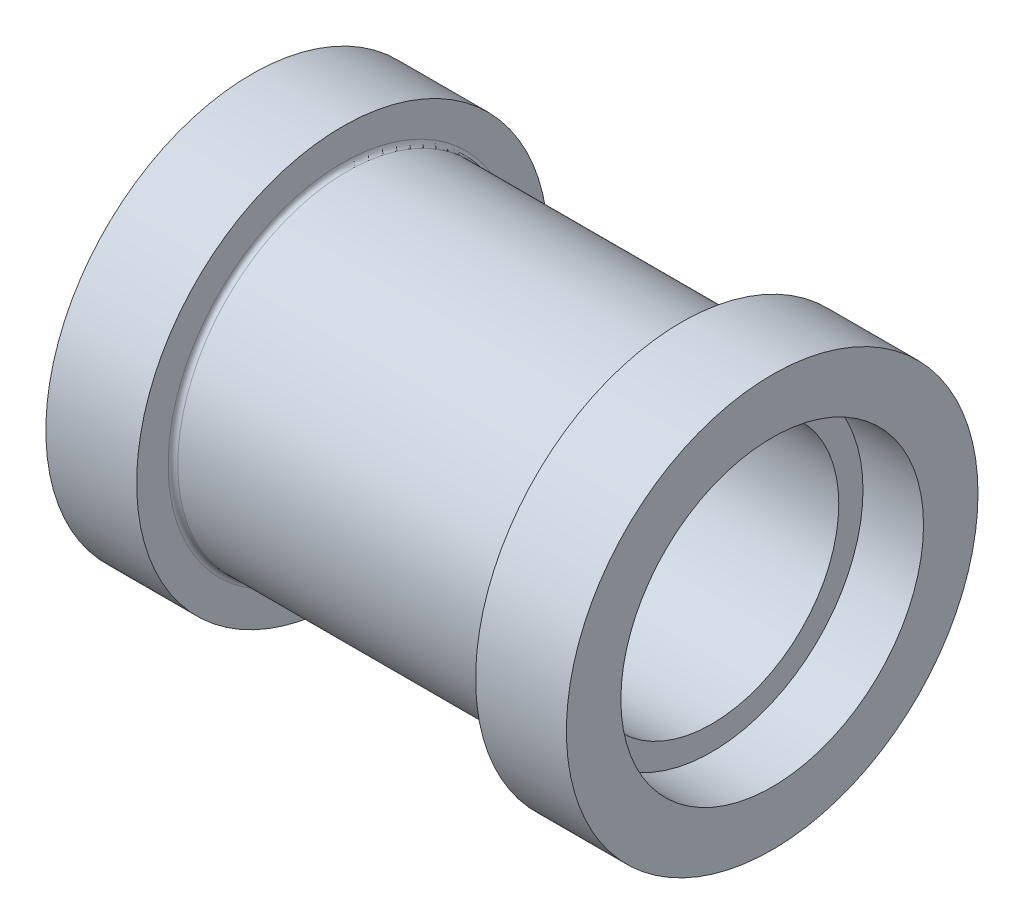
from build123d import *

# Parameters (mm, degrees)
SKETCH1_R           = 85
BOSS_EXTRUDE1_DEPTH = 215
CUT_EXTRUDE1_START  = 5
SKETCH2_R           = 110
SKETCH2_R_2         = 70
CUT_EXTRUDE1_DEPTH  = 140
FILLET1_R           = 2
SKETCH3_R           = 62.5
CUT_EXTRUDE2_DEPTH  = 25
CUT_EXTRUDE3_START  = -25
SKETCH4_R           = 62.5
CUT_EXTRUDE3_DEPTH  = 25
SKETCH5_R           = 52.5
CUT_EXTRUDE4_DEPTH  = 225.833271559


with BuildPart() as part:
    # Sketch1 → Boss-Extrude1 (new body)
    with BuildSketch(Plane(origin=(0, 0, 0), x_dir=(0, 0, -1), z_dir=(1, 0, 0))):
        Circle(SKETCH1_R)
    extrude(amount=BOSS_EXTRUDE1_DEPTH)

    # Sketch2 → Cut-Extrude1 (cut)
    with BuildSketch(Plane(origin=(172.5, 0, 0), x_dir=(0, 0, -1), z_dir=(1, 0, 0)).offset(CUT_EXTRUDE1_START)):
        Circle(SKETCH2_R)
        Circle(SKETCH2_R_2, mode=Mode.SUBTRACT)
    extrude(amount=-CUT_EXTRUDE1_DEPTH, mode=Mode.SUBTRACT)

    # Fillet1
    fillet1_edges = [part.edges().sort_by_distance(p)[0] for p in [
        (37.5, 0, 70),
        (177.5, 0, 70),
    ]]
    fillet(fillet1_edges, radius=FILLET1_R)

    # Sketch3 → Cut-Extrude2 (cut)
    with BuildSketch(Plane(origin=(215, 0, 0), x_dir=(0, 0, -1), z_dir=(1, 0, 0))):
        Circle(SKETCH3_R)
    extrude(amount=-CUT_EXTRUDE2_DEPTH, mode=Mode.SUBTRACT)

    # Sketch4 → Cut-Extrude3 (cut)
    with BuildSketch(Plane.ZY.offset(CUT_EXTRUDE3_START)):
        with Locations(Location((0, 0, 0), (0, 0, 180))):
            Circle(SKETCH4_R)
    extrude(amount=CUT_EXTRUDE3_DEPTH, mode=Mode.SUBTRACT)

    # Sketch5 → Cut-Extrude4 (cut, through all)
    with BuildSketch(Plane(origin=(190, 0, 0), x_dir=(0, 0, -1), z_dir=(1, 0, 0))):
        Circle(SKETCH5_R)
    extrude(amount=-CUT_EXTRUDE4_DEPTH, mode=Mode.SUBTRACT)


solid = part.part
